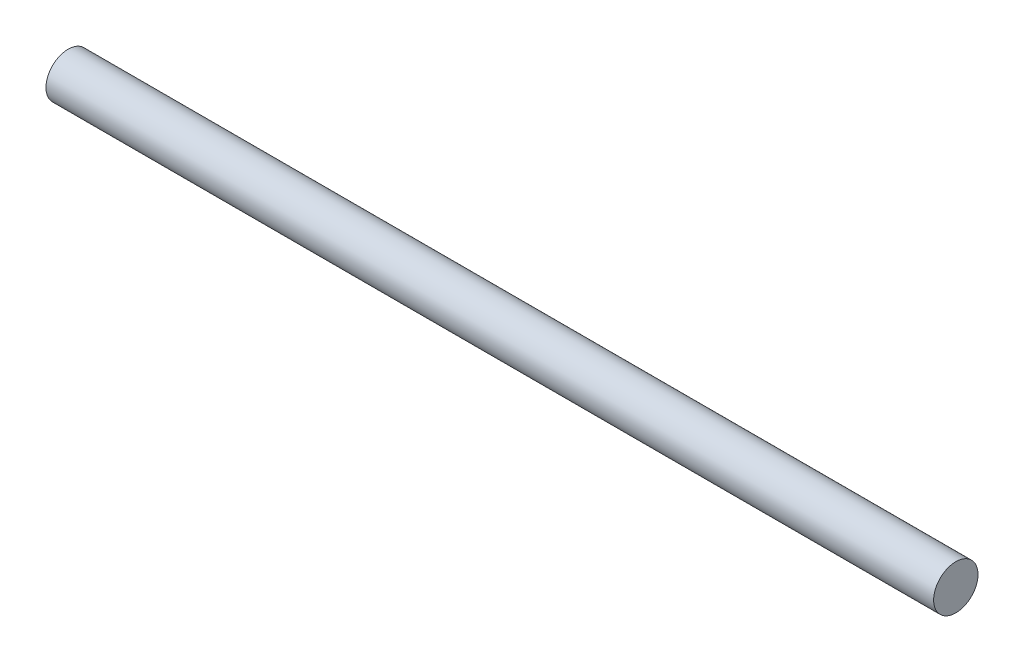
SolidWorks part; units mm, degrees
ref_plane "Front Plane" through (0, 0, 0) normal (0, 0, 1) x (1, 0, 0)
ref_plane "Top Plane" through (0, 0, 0) normal (0, 1, 0) x (1, 0, 0)
ref_plane "Right Plane" through (0, 0, 0) normal (1, 0, 0) x (0, 0, -1)
sketch "Sketch1" plane through (0, 0, 0) normal (1, 0, 0) x (0, 0, -1)
  circle A0 centre (0, 0) radius 20
  dimension "Durchmesser" = 40
extrude "Length" add sketch "Sketch1" along normal blind 800
